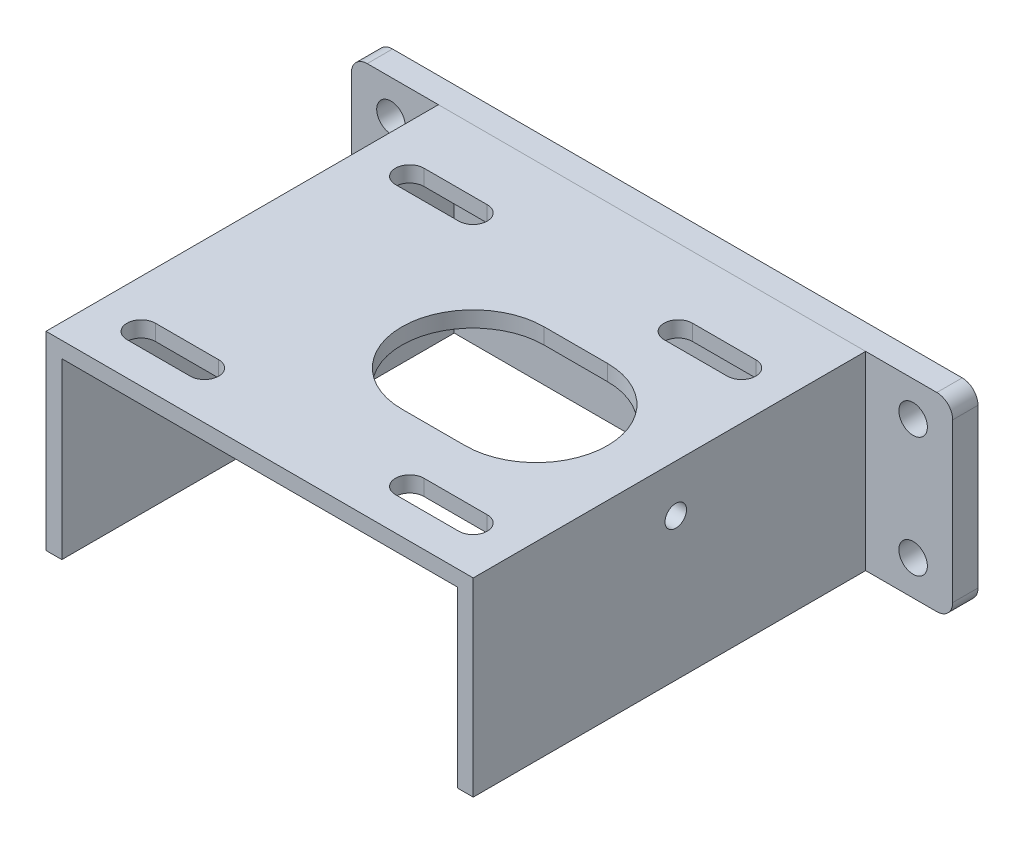
from build123d import *

# Parameters (mm, degrees)
SKETCH_1_W          = 190
SKETCH_1_H          = 60
EXTRUDE_1_DEPTH     = 8
SKETCH_2_R          = 4.5
CUT_EXTRUDE_1_DEPTH = 8
EXTRUDE_2_DEPTH     = 124
CUT_EXTRUDE_2_DEPTH = 150
FILLET_1_R          = 5
SKETCH_5_R          = 3.4
CUT_EXTRUDE_3_DEPTH = 212.495271815


with BuildPart() as part:
    # 草图1 → 凸台-拉伸1 (new body)
    with BuildSketch(Plane.XY):
        Rectangle(SKETCH_1_W, SKETCH_1_H)
    extrude(amount=EXTRUDE_1_DEPTH)

    # 草图2 → 切除-拉伸1 (cut)
    with BuildSketch(Plane.XY.offset(8)):
        with Locations((-82.5, 19)):
            Circle(SKETCH_2_R)
        with Locations((82.5, 19)):
            Circle(SKETCH_2_R)
        with Locations((82.5, -19)):
            Circle(SKETCH_2_R)
        with Locations((-82.5, -19)):
            Circle(SKETCH_2_R)
    extrude(amount=-CUT_EXTRUDE_1_DEPTH, mode=Mode.SUBTRACT)

    # 圆角1
    fillet_1_edges = [part.edges().sort_by_distance(p)[0] for p in [
        (95, -30, 4),
        (-95, -30, 4),
        (-95, 30, 4),
        (95, 30, 4),
    ]]
    fillet(fillet_1_edges, radius=FILLET_1_R)


with BuildPart() as body_2:
    # 草图3 → 凸台-拉伸2 (new body)
    with BuildSketch(Plane.XY.offset(8)):
        Polygon((-67.5, 30), (-67.5, -30), (-62.5, -30), (-62.5, 25), (62.5, 25), (62.5, -30), (67.5, -30), (67.5, 30), align=None)
    extrude(amount=EXTRUDE_2_DEPTH)

    # 草图4 → 切除-拉伸2 (cut)
    with BuildSketch(Plane(origin=(0, 30, 0), x_dir=(1, 0, 0), z_dir=(0, 1, 0))):
        with BuildLine():
            Line((-32.426406871, -112.5), (-52.426406871, -112.5))
            ThreePointArc((-52.426406871, -112.5), (-56.926406871, -117), (-52.426406871, -121.5))
            Line((-52.426406871, -121.5), (-32.426406871, -121.5))
            ThreePointArc((-32.426406871, -121.5), (-27.926406871, -117), (-32.426406871, -112.5))
        make_face()
        with BuildLine():
            Line((-32.426406871, -36.647186258), (-52.426406871, -36.647186258))
            ThreePointArc((-52.426406871, -36.647186258), (-56.926406871, -32.147186258), (-52.426406871, -27.647186258))
            Line((-52.426406871, -27.647186258), (-32.426406871, -27.647186258))
            ThreePointArc((-32.426406871, -27.647186258), (-27.926406871, -32.147186258), (-32.426406871, -36.647186258))
        make_face()
        with BuildLine():
            Line((32.426406871, -27.647186258), (52.426406871, -27.647186258))
            ThreePointArc((52.426406871, -27.647186258), (56.926406871, -32.147186258), (52.426406871, -36.647186258))
            Line((52.426406871, -36.647186258), (32.426406871, -36.647186258))
            ThreePointArc((32.426406871, -36.647186258), (27.926406871, -32.147186258), (32.426406871, -27.647186258))
        make_face()
        with BuildLine():
            Line((32.426406871, -112.5), (52.426406871, -112.5))
            ThreePointArc((52.426406871, -112.5), (56.926406871, -117), (52.426406871, -121.5))
            Line((52.426406871, -121.5), (32.426406871, -121.5))
            ThreePointArc((32.426406871, -121.5), (27.926406871, -117), (32.426406871, -112.5))
        make_face()
        with BuildLine():
            Line((10, -52.073593129), (30, -52.073593129))
            ThreePointArc((30, -52.073593129), (52.5, -74.573593129), (30, -97.073593129))
            Line((30, -97.073593129), (10, -97.073593129))
            ThreePointArc((10, -97.073593129), (-12.5, -74.573593129), (10, -52.073593129))
        make_face()
    extrude(amount=-CUT_EXTRUDE_2_DEPTH, mode=Mode.SUBTRACT)

    # 草图5 → 切除-拉伸3 (cut, through all)
    with BuildSketch(Plane(origin=(67.5, 0, 0), x_dir=(0, 0, -1), z_dir=(1, 0, 0))):
        with Locations((-68, 15)):
            Circle(SKETCH_5_R)
    extrude(amount=-CUT_EXTRUDE_3_DEPTH, mode=Mode.SUBTRACT)


solid = Compound([part.part, body_2.part])
